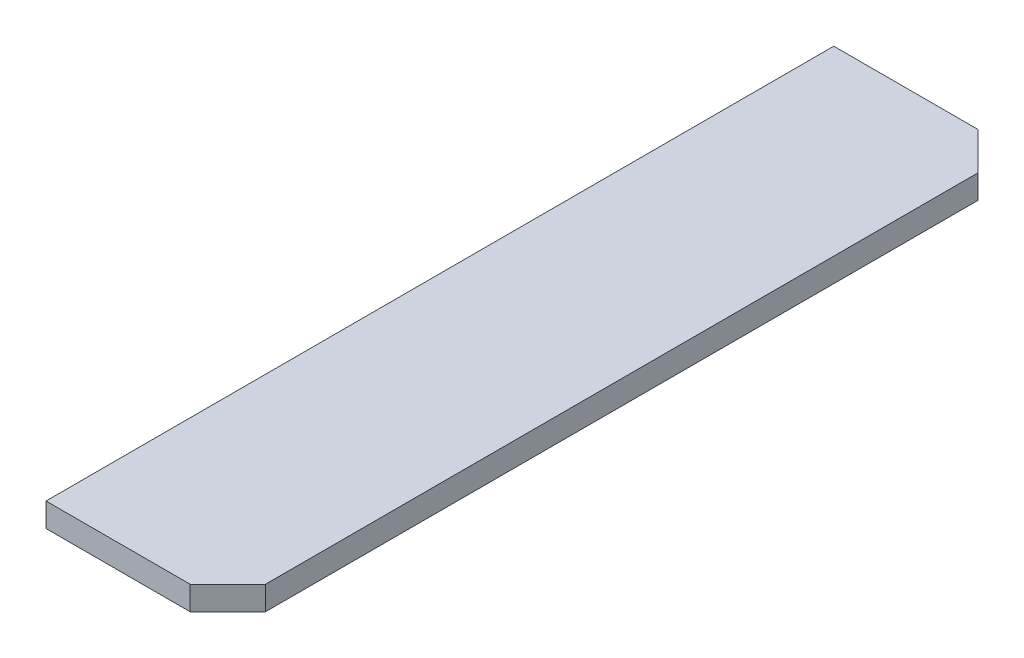
SolidWorks part; units mm, degrees
material "普通碳钢"
ref_plane "Front Plane" through (0, 0, 0) normal (0, 0, 1) x (1, 0, 0)
ref_plane "Top Plane" through (0, 0, 0) normal (0, 1, 0) x (1, 0, 0)
ref_plane "Right Plane" through (0, 0, 0) normal (1, 0, 0) x (0, 0, -1)
sketch "Sketch3" plane through (0, 0, 0) normal (0, 1, 0) x (1, 0, 0)
  line L0 (19.556, 140.716) -> (35.306, 124.966)
  line L1 (-40.894, 140.716) -> (19.556, 140.716)
  line L2 (-40.894, 140.716) -> (-40.894, -189.484)
  line L3 (-40.894, -189.484) -> (19.556, -189.484)
  line L4 (35.306, 124.966) -> (35.306, -173.734)
  line L5 (35.306, -173.734) -> (19.556, -189.484)
  circle A0 centre (0, 0) radius 14.224 construction
  point P1 (35.306, -189.484)
  point P3 (35.306, 140.716)
  dimension "D3" = 35.306
  dimension "D7" = 28.448
  dimension "D1" = 76.2
  dimension "D2" = 330.2
  dimension "D4" = 140.716
extrude "Boss-Extrude1" add sketch "Sketch3" along normal mid plane 10
